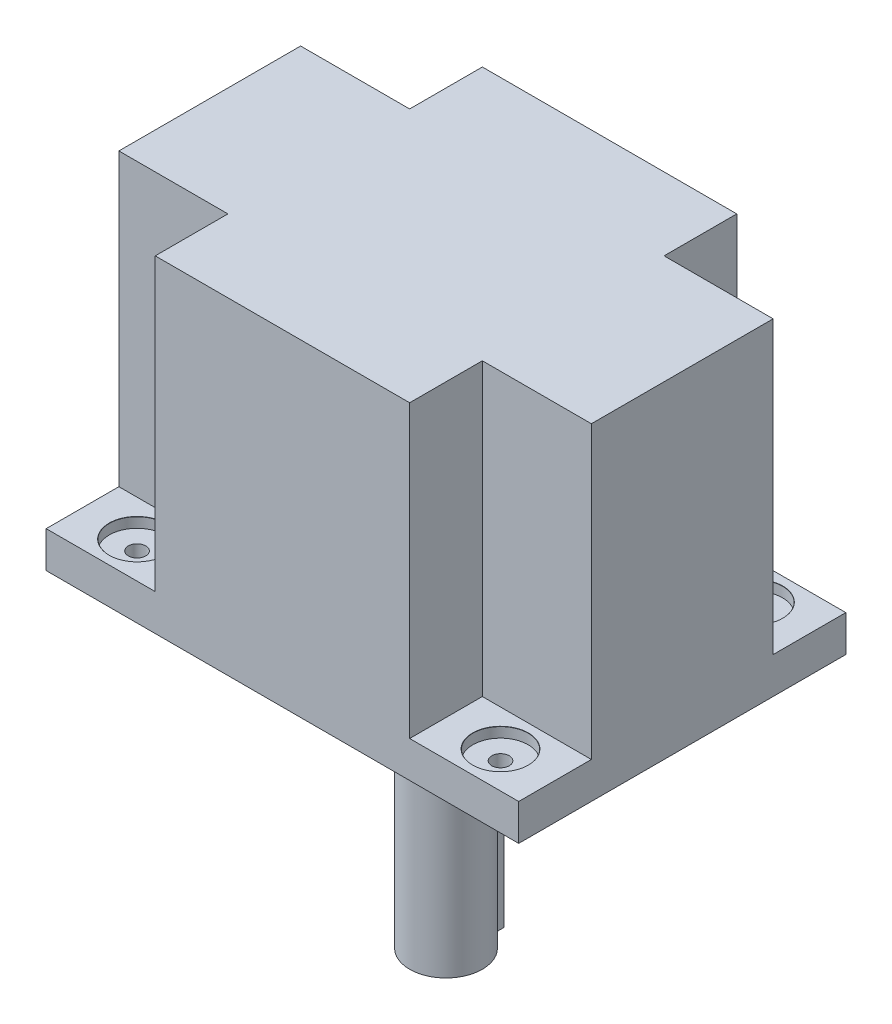
from build123d import *

# Parameters (mm, degrees)
SKETCH1_W                              = 65
SKETCH1_H                              = 45
BOSS_EXTRUDE1_DEPTH                    = 45
SKETCH2_W                              = 15
SKETCH2_H                              = 10
CUT_EXTRUDE1_DEPTH                     = 40
SKETCH3_R                              = 5
BOSS_EXTRUDE2_DEPTH                    = 40
BOSS_EXTRUDE3_START                    = -40
BOSS_EXTRUDE3_DEPTH                    = 40
SKETCH5_R                              = 15
BOSS_EXTRUDE4_DEPTH                    = 2
CBORE_FOR_M2_HEX_CAP_SCREW2_AT_2_COUNT = 2
CBORE_FOR_M2_HEX_CAP_SCREW2_AT_2_PITCH = 50
CBORE_FOR_M2_HEX_CAP_SCREW2_AT_3_COUNT = 2
CBORE_FOR_M2_HEX_CAP_SCREW2_AT_3_PITCH = 35
CBORE_FOR_M2_HEX_CAP_SCREW2_AT_4_COUNT = 2
CBORE_FOR_M2_HEX_CAP_SCREW2_AT_4_PITCH = 61.032778079


with BuildPart() as part:
    # Sketch1 → Boss-Extrude1 (new body)
    with BuildSketch(Plane(origin=(0, 0, 0), x_dir=(1, 0, 0), z_dir=(0, 1, 0))):
        Rectangle(SKETCH1_W, SKETCH1_H)
    extrude(amount=BOSS_EXTRUDE1_DEPTH)

    # Sketch2 → Cut-Extrude1 (cut)
    with BuildSketch(Plane(origin=(0, 45, 0), x_dir=(1, 0, 0), z_dir=(0, 1, 0))):
        with Locations((-25, 17.5)):
            Rectangle(SKETCH2_W, SKETCH2_H)
        with Locations((-25, -17.5)):
            Rectangle(SKETCH2_W, SKETCH2_H)
        with Locations((25, -17.5)):
            Rectangle(SKETCH2_W, SKETCH2_H)
        with Locations((25, 17.5)):
            Rectangle(SKETCH2_W, SKETCH2_H)
    extrude(amount=-CUT_EXTRUDE1_DEPTH, mode=Mode.SUBTRACT)

    # Sketch3 → Boss-Extrude2 (add)
    with BuildSketch(Plane.XZ):
        with Locations(Location((0, 0, 0), (0, 0, 270))):
            Circle(SKETCH3_R)
    extrude(amount=BOSS_EXTRUDE2_DEPTH)

    # Sketch4 → Boss-Extrude3 (add)
    with BuildSketch(Plane.XZ.offset(40).offset(BOSS_EXTRUDE3_START)):
        with BuildLine():
            ThreePointArc((1.5, -4.769696007), (0.758788496, -4.942088629), (0, -5))
            ThreePointArc((0, -5), (-0.758788496, -4.942088629), (-1.5, -4.769696007))
            Line((-1.5, -4.769696007), (-1.5, -6.5))
            Line((-1.5, -6.5), (1.5, -6.5))
            Line((1.5, -6.5), (1.5, -4.769696007))
        make_face()
    extrude(amount=BOSS_EXTRUDE3_DEPTH)

    # Sketch5 → Boss-Extrude4 (add)
    with BuildSketch(Plane.XZ):
        with Locations(Location((0, 0, 0), (0, 0, 270))):
            Circle(SKETCH5_R)
    extrude(amount=BOSS_EXTRUDE4_DEPTH)

    # Sketch8 → CBORE for M2 Hex Cap Screw1 (revolve, cut)
    with BuildSketch(Plane(origin=(0, -40, 0), x_dir=(0, 0, -1), z_dir=(1, 0, 0))):
        Polygon((0, 0), (0, 5.721032743), (1.2, 5), (1.2, 1.4), (3.8095, 1.4), (3.8095, 0.025), (3.8345, 0), align=None)
    revolve(axis=Axis((0, -46.35, 0), (0, 1, 0)), mode=Mode.SUBTRACT)

    # Sketch12 → CBORE for M2 Hex Cap Screw2 (revolve, cut)
    with BuildSketch(Plane(origin=(-25, 5, -17.5), x_dir=(0, 0, 1), z_dir=(1, 0, 0))):
        Polygon((0, 0), (0, 10.721032743), (1.2, 10), (1.2, 1.4), (3.8095, 1.4), (3.8095, 0.025), (3.8345, 0), align=None)
    cbore_for_m2_hex_cap_screw2 = revolve(axis=Axis((-25, 11.35, -17.5), (0, -1, 0)), mode=Mode.SUBTRACT)

    # CBORE for M2 Hex Cap Screw2 at 2: CBORE for M2 Hex Cap Screw2 ×2
    with Locations(*[(i * CBORE_FOR_M2_HEX_CAP_SCREW2_AT_2_PITCH, 0, 0) for i in range(1, CBORE_FOR_M2_HEX_CAP_SCREW2_AT_2_COUNT)]):
        add(cbore_for_m2_hex_cap_screw2, mode=Mode.SUBTRACT)

    # CBORE for M2 Hex Cap Screw2 at 3: CBORE for M2 Hex Cap Screw2 ×2
    with Locations(*[(0, 0, i * CBORE_FOR_M2_HEX_CAP_SCREW2_AT_3_PITCH) for i in range(1, CBORE_FOR_M2_HEX_CAP_SCREW2_AT_3_COUNT)]):
        add(cbore_for_m2_hex_cap_screw2, mode=Mode.SUBTRACT)

    # CBORE for M2 Hex Cap Screw2 at 4: CBORE for M2 Hex Cap Screw2 ×2
    with Locations(*[Vector(0.8192319205190405, 0, 0.5734623443633283) * (i * CBORE_FOR_M2_HEX_CAP_SCREW2_AT_4_PITCH) for i in range(1, CBORE_FOR_M2_HEX_CAP_SCREW2_AT_4_COUNT)]):
        add(cbore_for_m2_hex_cap_screw2, mode=Mode.SUBTRACT)


solid = part.part
